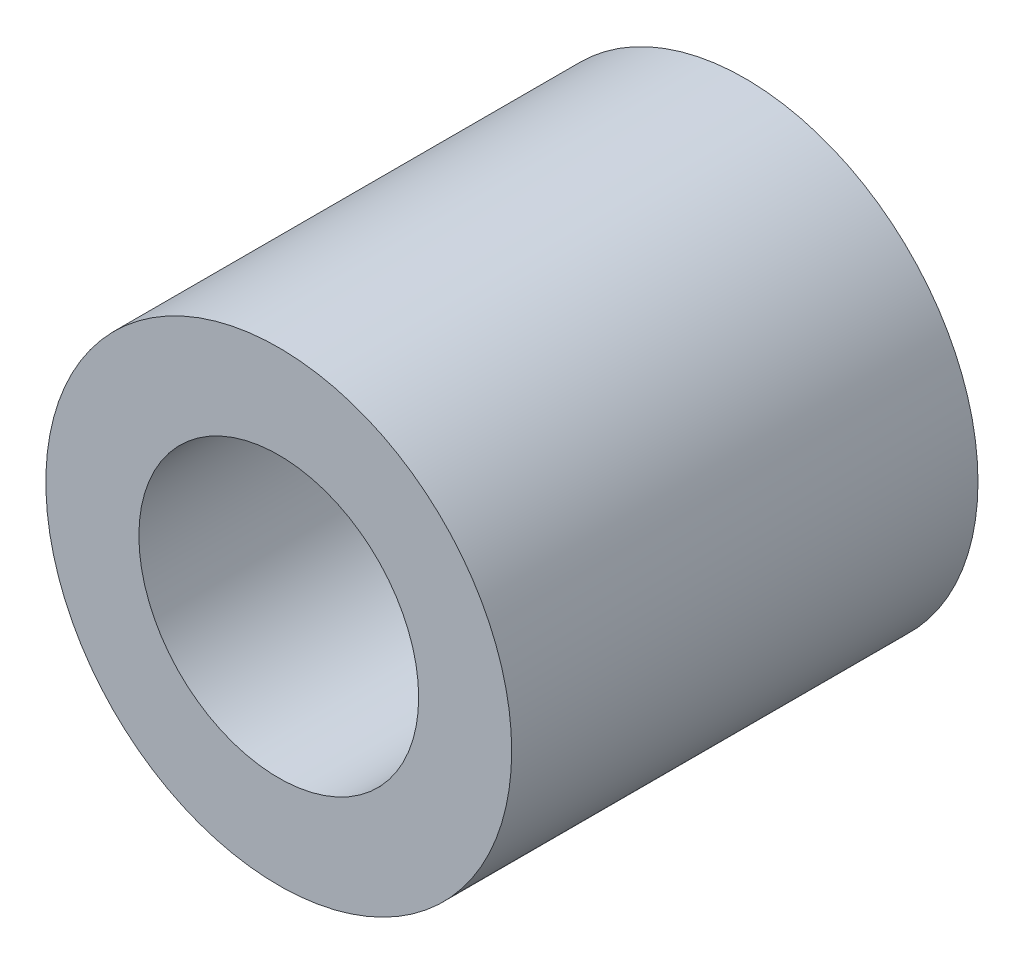
from build123d import *

# Parameters (mm, degrees)
SKETCH1_R           = 4.995
SKETCH1_R_2         = 3
BOSS_EXTRUDE1_DEPTH = 10


with BuildPart() as part:
    # Sketch1 → Boss-Extrude1 (new body)
    with BuildSketch(Plane.XY):
        Circle(SKETCH1_R)
        Circle(SKETCH1_R_2, mode=Mode.SUBTRACT)
    extrude(amount=BOSS_EXTRUDE1_DEPTH)


solid = part.part
